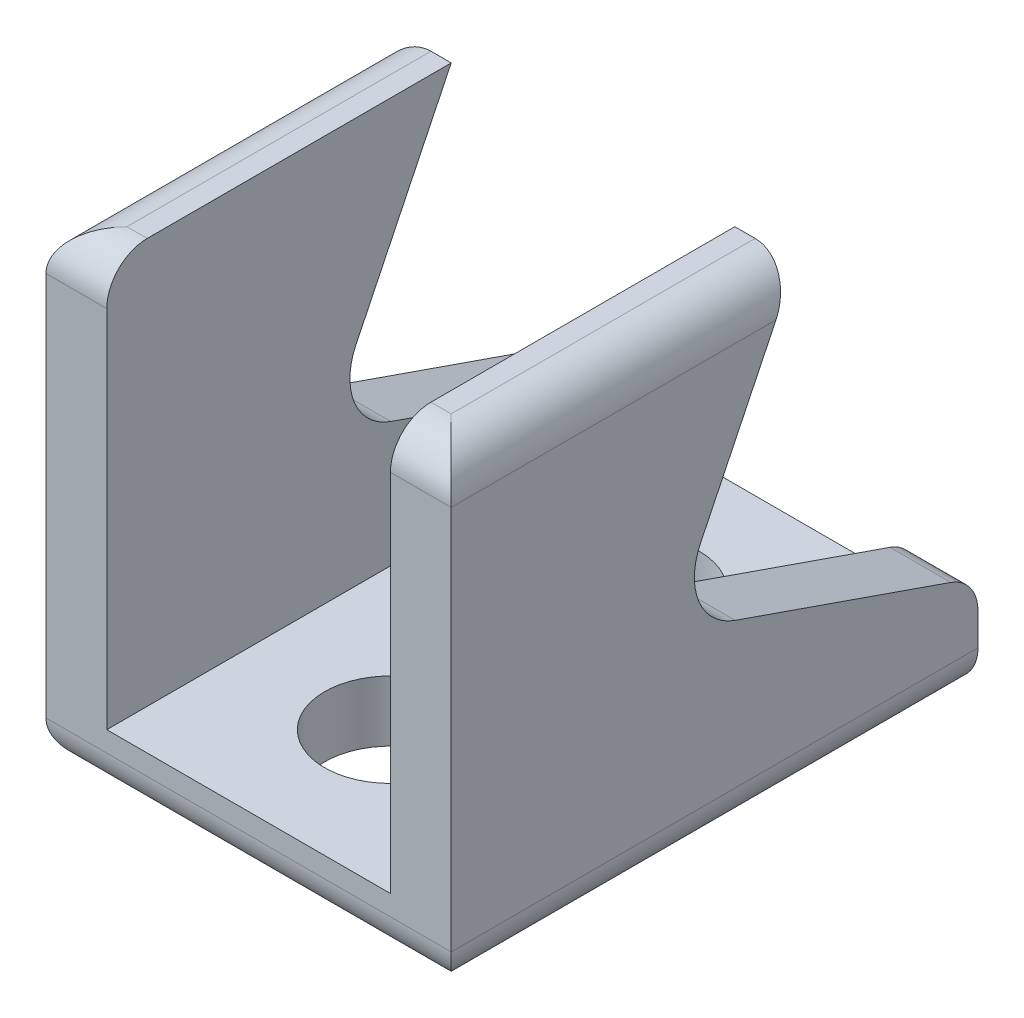
from build123d import *

# Parameters (mm, degrees)
EXTRUDE_1_DEPTH     = 10
SKETCH_2_W          = 26
SKETCH_2_H          = 20
CUT_EXTRUDE_1_DEPTH = 7
CUT_EXTRUDE_2_REACH = 38.125
SKETCH_3_R          = 3.25
FILLET_3_R          = 2


with BuildPart() as part:
    # 草图1 → 凸台-拉伸1 (new, symmetric)
    with BuildSketch(Plane(origin=(0, 0, 0), x_dir=(0, 0, -1), z_dir=(1, 0, 0))):
        with BuildLine():
            Line((17, 23), (0, 23))
            Line((0, 23), (0, 0))
            Line((0, 0), (26, 0))
            Line((26, 0), (26, 5))
            Line((26, 5), (14.014940421, 9.166334948))
            ThreePointArc((14.014940421, 9.166334948), (12.227975796, 10.852881082), (12.300632982, 13.308975821))
            Line((12.300632982, 13.308975821), (17, 23))
        make_face()
    extrude(amount=EXTRUDE_1_DEPTH, both=True)

    # 草图2 → 切除-拉伸1 (cut, symmetric)
    with BuildSketch(Plane(origin=(0, 0, 0), x_dir=(0, 0, -1), z_dir=(1, 0, 0))):
        with Locations((13, 13)):
            Rectangle(SKETCH_2_W, SKETCH_2_H)
    extrude(amount=CUT_EXTRUDE_1_DEPTH, both=True, mode=Mode.SUBTRACT)

    # 草图3 → 切除-拉伸2 (cut, up to next)
    with BuildSketch(Plane.XZ, mode=Mode.PRIVATE) as cut_extrude_2_sk1:
        with Locations(Location((0, -7, 0), (0, 0, 270))):
            Circle(SKETCH_3_R)
    cut_extrude_2_tool1 = extrude(cut_extrude_2_sk1.sketch, amount=-CUT_EXTRUDE_2_REACH, mode=Mode.PRIVATE) & part.part
    # 草图3 → 切除-拉伸2 (cut, up to next)
    with BuildSketch(Plane.XZ, mode=Mode.PRIVATE) as cut_extrude_2_sk2:
        with Locations(Location((0, -19, 0), (0, 0, 270))):
            Circle(SKETCH_3_R)
    cut_extrude_2_tool2 = extrude(cut_extrude_2_sk2.sketch, amount=-CUT_EXTRUDE_2_REACH, mode=Mode.PRIVATE) & part.part
    add(cut_extrude_2_tool1.solids().sort_by_distance((0, 0, -7))[0], mode=Mode.SUBTRACT)
    add(cut_extrude_2_tool2.solids().sort_by_distance((0, 0, -19))[0], mode=Mode.SUBTRACT)

    # 圆角3
    fillet_3_edges = [part.edges().sort_by_distance(p)[0] for p in [
        (-10, 23, -8.5),
        (10, 23, -8.5),
        (8.5, 5, -26),
        (0, 0, 0),
        (8.5, 23, 0),
        (10, 0, -13),
        (-8.5, 5, -26),
        (-8.5, 23, 0),
        (-10, 0, -13),
    ]]
    fillet(fillet_3_edges, radius=FILLET_3_R)


solid = part.part
